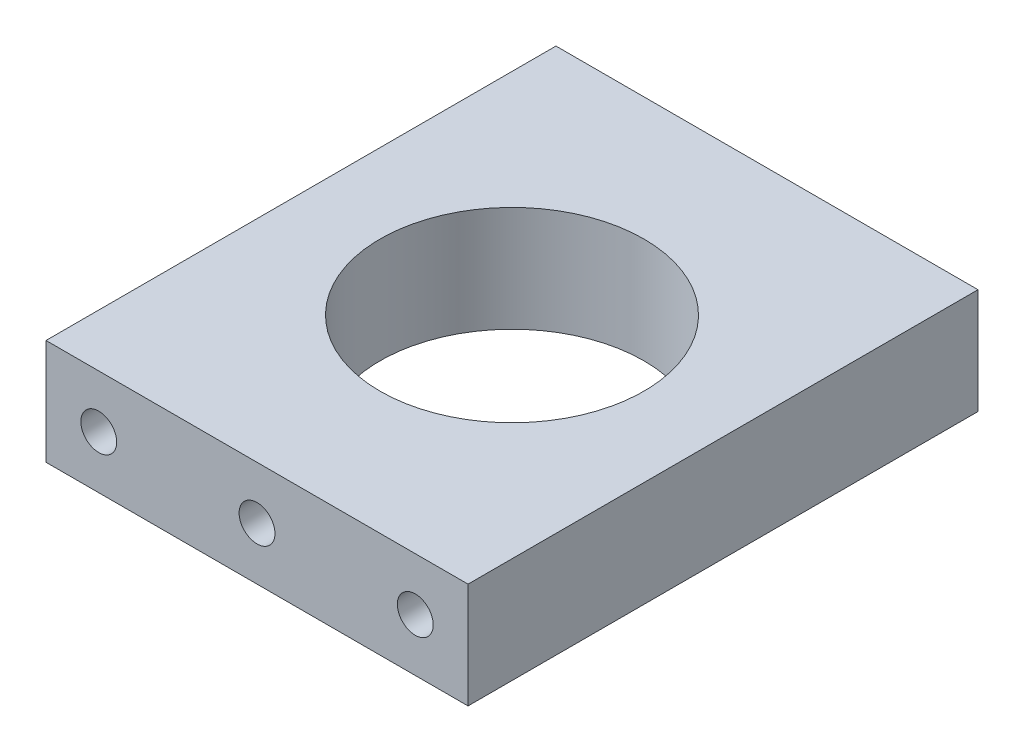
from build123d import *

# Parameters (mm, degrees)
SKETCH_1_W                   = 120
SKETCH_1_H                   = 145
SKETCH_1_R                   = 37.5
EXTRUDE_1_DEPTH              = 30
HOLE_WIZARD_M10_1_D          = 8.5
HOLE_WIZARD_M10_1_DEPTH      = 24.5
HOLE_WIZARD_M10_1_TIP        = 2.553657631
HOLE_WIZARD_M12_1_AT_2_COUNT = 2
HOLE_WIZARD_M12_1_AT_2_PITCH = 45
HOLE_WIZARD_M12_1_AT_3_COUNT = 2
HOLE_WIZARD_M12_1_AT_3_PITCH = 90


with BuildPart() as part:
    # 草图1 → 凸台-拉伸1 (new body)
    with BuildSketch(Plane(origin=(0, 0, 0), x_dir=(1, 0, 0), z_dir=(0, 1, 0))):
        Rectangle(SKETCH_1_W, SKETCH_1_H)
        with Locations(Location((0, 0, 0), (0, 0, 270))):
            Circle(SKETCH_1_R, mode=Mode.SUBTRACT)
    extrude(amount=EXTRUDE_1_DEPTH)

    # M10 螺纹孔1
    with Locations(Plane(origin=(0, 0, 0), x_dir=(-1, 0, 0), z_dir=(0, -1, 0))):
        with Locations((-32.880465325, -32.880465325), (-44.915550922, -12.035085597), (-44.915550922, 12.035085597), (-32.880465325, 32.880465325), (32.880465325, 32.880465325), (44.915550922, 12.035085597), (44.915550922, -12.035085597), (32.880465325, -32.880465325)):
            Hole(HOLE_WIZARD_M10_1_D / 2, depth=HOLE_WIZARD_M10_1_DEPTH)
            with Locations((0, 0, -(HOLE_WIZARD_M10_1_DEPTH + HOLE_WIZARD_M10_1_TIP / 2))):  # 118° drill point
                Cone(0, HOLE_WIZARD_M10_1_D / 2, HOLE_WIZARD_M10_1_TIP, mode=Mode.SUBTRACT)

    # 草图5 → M12 螺纹孔1 (revolve, cut)
    with BuildSketch(Plane(origin=(-45, 15, -72.5), x_dir=(0, 1, 0), z_dir=(1, 0, 0))):
        Polygon((0, 0), (0, 32.314389157), (5.1, 29.25), (5.1, 0), align=None)
    hole_wizard_m12_1 = revolve(axis=Axis((-45, 15, -78.85), (0, 0, 1)), mode=Mode.SUBTRACT)

    # M12 螺纹孔1 at 2: M12 螺纹孔1 ×2
    with Locations(*[(i * HOLE_WIZARD_M12_1_AT_2_PITCH, 0, 0) for i in range(1, HOLE_WIZARD_M12_1_AT_2_COUNT)]):
        add(hole_wizard_m12_1, mode=Mode.SUBTRACT)

    # M12 螺纹孔1 at 3: M12 螺纹孔1 ×2
    with Locations(*[(i * HOLE_WIZARD_M12_1_AT_3_PITCH, 0, 0) for i in range(1, HOLE_WIZARD_M12_1_AT_3_COUNT)]):
        add(hole_wizard_m12_1, mode=Mode.SUBTRACT)

    # 镜向1: M12 螺纹孔1 across plane
    add(hole_wizard_m12_1.mirror(Plane.XY), mode=Mode.SUBTRACT)

    # 镜向1 copy 1 sketch → 镜向1 copy 1 (revolve, cut)
    with BuildSketch(Plane(origin=(0, 15, 72.5), x_dir=(0, 1, 0), z_dir=(1, 0, 0))):
        Polygon((0, 0), (0, -32.314389157), (5.1, -29.25), (5.1, 0), align=None)
    revolve(axis=Axis((0, 15, 78.85), (0, 0, 1)), mode=Mode.SUBTRACT)

    # 镜向1 copy 2 sketch → 镜向1 copy 2 (revolve, cut)
    with BuildSketch(Plane(origin=(45, 15, 72.5), x_dir=(0, 1, 0), z_dir=(1, 0, 0))):
        Polygon((0, 0), (0, -32.314389157), (5.1, -29.25), (5.1, 0), align=None)
    revolve(axis=Axis((45, 15, 78.85), (0, 0, 1)), mode=Mode.SUBTRACT)


solid = part.part
